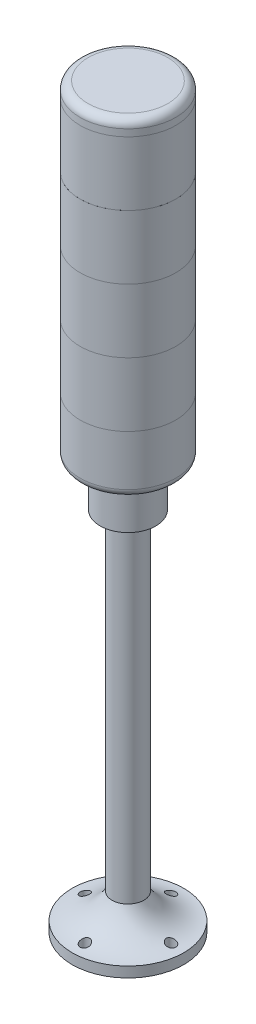
from build123d import *

# Parameters (mm, degrees)
SKETCH_1_R                     = 30
EXTRUDE_1_DEPTH                = 20
SKETCH_2_R                     = 30
EXTRUDE_2_DEPTH                = 40
SKETCH_3_R                     = 30
EXTRUDE_3_DEPTH                = 40
SKETCH_4_R                     = 30
EXTRUDE_4_DEPTH                = 40
SKETCH_5_R                     = 30
EXTRUDE_5_DEPTH                = 9.35
SKETCH_6_R                     = 30
EXTRUDE_6_DEPTH                = 9.35
SKETCH_7_R                     = 30
EXTRUDE_7_DEPTH                = 27.2
SKETCH_8_R                     = 17.5
EXTRUDE_8_DEPTH                = 27.2
FILLET_1_R                     = 5
SKETCH_9_R                     = 10
EXTRUDE_9_DEPTH                = 207
FILLET_2_R                     = 5
FILLET_3_R                     = 5
SKETCH_10_R                    = 35
EXTRUDE_10_DEPTH               = 22.5
HOLE_WIZARD_6_0_6_2_AT_2_COUNT = 2
HOLE_WIZARD_6_0_6_2_AT_2_PITCH = 54
HOLE_WIZARD_6_0_6_2_AT_3_COUNT = 2
HOLE_WIZARD_6_0_6_2_AT_3_PITCH = 38.183766184
HOLE_WIZARD_6_0_6_2_AT_4_COUNT = 2
HOLE_WIZARD_6_0_6_2_AT_4_PITCH = 38.183766184


with BuildPart() as part:
    # 草图1 → 凸台-拉伸1 (new, symmetric)
    with BuildSketch(Plane(origin=(0, 0, 0), x_dir=(1, 0, 0), z_dir=(0, 1, 0))):
        with Locations(Location((0, 0, 0), (0, 0, 270))):
            Circle(SKETCH_1_R)
    extrude(amount=EXTRUDE_1_DEPTH, both=True)


with BuildPart() as body_2:
    # 草图2 → 凸台-拉伸2 (new body)
    with BuildSketch(Plane.XZ.offset(20)):
        with Locations(Location((0, 0, 0), (0, 0, 270))):
            Circle(SKETCH_2_R)
    extrude(amount=EXTRUDE_2_DEPTH)


with BuildPart() as body_3:
    # 草图3 → 凸台-拉伸3 (new body)
    with BuildSketch(Plane.XZ.offset(60)):
        with Locations(Location((0, 0, 0), (0, 0, 270))):
            Circle(SKETCH_3_R)
    extrude(amount=EXTRUDE_3_DEPTH)


with BuildPart() as body_4:
    # 草图4 → 凸台-拉伸4 (new body)
    with BuildSketch(Plane.XZ.offset(100)):
        with Locations(Location((0, 0, 0), (0, 0, 270))):
            Circle(SKETCH_4_R)
    extrude(amount=EXTRUDE_4_DEPTH)


with BuildPart() as body_5:
    # 草图5 → 凸台-拉伸5 (new body)
    with BuildSketch(Plane(origin=(0, 20, 0), x_dir=(1, 0, 0), z_dir=(0, 1, 0))):
        with Locations(Location((0, 0, 0), (0, 0, 270))):
            Circle(SKETCH_5_R)
    extrude(amount=EXTRUDE_5_DEPTH)

    # 圆角1
    fillet_1_edges = [body_5.edges().sort_by_distance(p)[0] for p in [
        (0, 29.35, -30),
    ]]
    fillet(fillet_1_edges, radius=FILLET_1_R)


with BuildPart() as body_6:
    # 草图6 → 凸台-拉伸6 (new body)
    with BuildSketch(Plane.XZ.offset(140)):
        with Locations(Location((0, 0, 0), (0, 0, 270))):
            Circle(SKETCH_6_R)
    extrude(amount=EXTRUDE_6_DEPTH)

    # 草图7 → 凸台-拉伸7 (add)
    with BuildSketch(Plane.XZ.offset(149.35)):
        with Locations(Location((0, 0, 0), (0, 0, 270))):
            Circle(SKETCH_7_R)
    extrude(amount=EXTRUDE_7_DEPTH)

    # 草图8 → 凸台-拉伸8 (add)
    with BuildSketch(Plane.XZ.offset(176.55)):
        with Locations(Location((0, 0, 0), (0, 0, 270))):
            Circle(SKETCH_8_R)
    extrude(amount=EXTRUDE_8_DEPTH)

    # 草图9 → 凸台-拉伸9 (add)
    with BuildSketch(Plane.XZ.offset(203.75)):
        with Locations(Location((0, 0, 0), (0, 0, 270))):
            Circle(SKETCH_9_R)
    extrude(amount=EXTRUDE_9_DEPTH)

    # 圆角2
    fillet_2_edges = [body_6.edges().sort_by_distance(p)[0] for p in [
        (0, -176.55, 17.5),
    ]]
    fillet(fillet_2_edges, radius=FILLET_2_R)

    # 圆角3
    fillet_3_edges = [body_6.edges().sort_by_distance(p)[0] for p in [
        (0, -176.55, 30),
    ]]
    fillet(fillet_3_edges, radius=FILLET_3_R)

    # 草图10 → 凸台-拉伸10 (add)
    with BuildSketch(Plane.XZ.offset(410.75)):
        with Locations(Location((0, 0, 0), (0, 0, 90))):
            Circle(SKETCH_10_R)
    extrude(amount=EXTRUDE_10_DEPTH)

    # 草图11 → 切除-旋转1 (revolve, cut)
    with BuildSketch(Plane(origin=(0, 0, 0), x_dir=(0, 0, -1), z_dir=(1, 0, 0))):
        with BuildLine():
            Line((10, -410.75), (35, -410.75))
            Line((35, -410.75), (35, -426.75))
            ThreePointArc((35, -426.75), (20.205474893, -422.33519548), (10, -410.75))
        make_face()
    revolve(axis=Axis((0, -433.25, 0), (0, 1, 0)), mode=Mode.SUBTRACT)

    # 草图15 → Ø6.0 (6) 直径孔2 (revolve, cut)
    with BuildSketch(Plane(origin=(0, -433.25, 27), x_dir=(0, 0, -1), z_dir=(1, 0, 0))):
        Polygon((0, 0), (0, 36.802581857), (3, 35), (3, 0), align=None)
    hole_wizard_6_0_6_2 = revolve(axis=Axis((0, -439.6, 27), (0, 1, 0)), mode=Mode.SUBTRACT)

    # Ø6.0 (6) 直径孔2 at 2: Ø6.0 (6) 直径孔2 ×2
    with Locations(*[(0, 0, -i * HOLE_WIZARD_6_0_6_2_AT_2_PITCH) for i in range(1, HOLE_WIZARD_6_0_6_2_AT_2_COUNT)]):
        add(hole_wizard_6_0_6_2, mode=Mode.SUBTRACT)

    # Ø6.0 (6) 直径孔2 at 3: Ø6.0 (6) 直径孔2 ×2
    with Locations(*[Vector(-0.7071067811865476, 0, -0.7071067811865476) * (i * HOLE_WIZARD_6_0_6_2_AT_3_PITCH) for i in range(1, HOLE_WIZARD_6_0_6_2_AT_3_COUNT)]):
        add(hole_wizard_6_0_6_2, mode=Mode.SUBTRACT)

    # Ø6.0 (6) 直径孔2 at 4: Ø6.0 (6) 直径孔2 ×2
    with Locations(*[Vector(0.7071067811865476, 0, -0.7071067811865476) * (i * HOLE_WIZARD_6_0_6_2_AT_4_PITCH) for i in range(1, HOLE_WIZARD_6_0_6_2_AT_4_COUNT)]):
        add(hole_wizard_6_0_6_2, mode=Mode.SUBTRACT)


solid = Compound([part.part, body_2.part, body_3.part, body_4.part, body_5.part, body_6.part])
